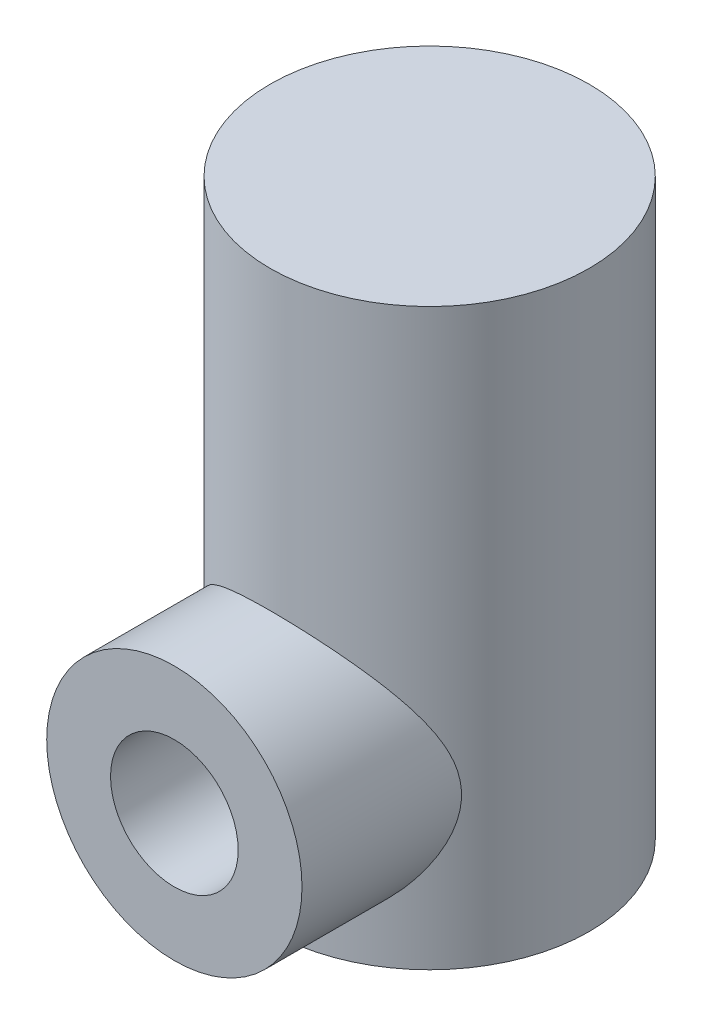
from build123d import *

# Parameters (mm, degrees)
SKETCH_1_R           = 4
SKETCH_1_R_2         = 2
EXTRUDE_1_DEPTH      = 8
EXTRUDE_2_DEPTH      = 12
EXTRUDE_2_DEPTH_BACK = 6
SKETCH_3_R           = 5


with BuildPart() as part:
    # 草图1 → 凸台-拉伸1 (new body)
    with BuildSketch(Plane.XY):
        with Locations((2.360745364, -1.287337305)):
            Circle(SKETCH_1_R)
        with Locations((2.360745364, -1.287337305)):
            Circle(SKETCH_1_R_2, mode=Mode.SUBTRACT)
    extrude(amount=EXTRUDE_1_DEPTH)

    # 草图3 → 凸台-拉伸2 (add, two sides: drawn at the far end of the back side and taken through both)
    with BuildSketch(Plane(origin=(0, 0, 0), x_dir=(1, 0, 0), z_dir=(0, 1, 0)).offset(-EXTRUDE_2_DEPTH_BACK)):
        with Locations(Location((2.360745364, 0, 0), (0, 0, 270))):
            Circle(SKETCH_3_R)
    extrude(amount=EXTRUDE_2_DEPTH + EXTRUDE_2_DEPTH_BACK)


solid = part.part
